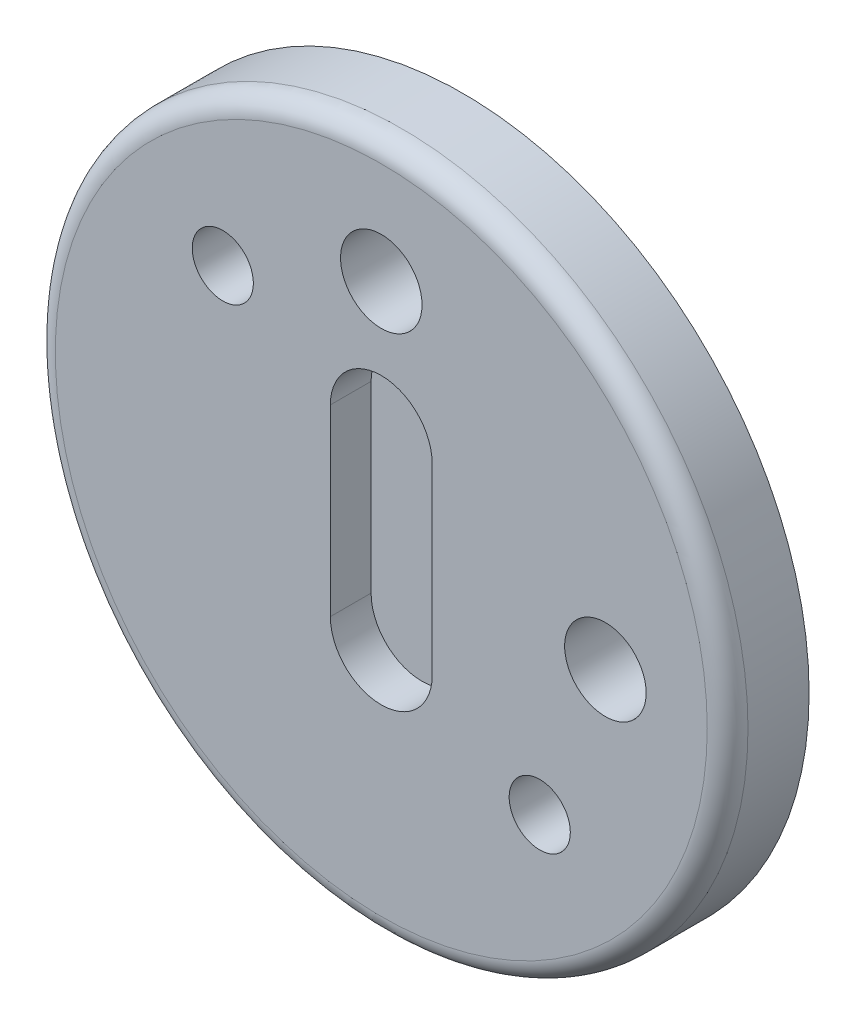
SolidWorks part; units mm, degrees
ref_plane "Front Plane" through (0, 0, 0) normal (0, 0, 1) x (1, 0, 0)
ref_plane "Top Plane" through (0, 0, 0) normal (0, 1, 0) x (1, 0, 0)
ref_plane "Right Plane" through (0, 0, 0) normal (1, 0, 0) x (0, 0, -1)
other "Configuration Table"
sketch "Sketch1" plane through (0, 0, 0) normal (0, 0, 1) x (1, 0, 0)
  circle A0 centre (0, 0) radius 17
  dimension "D1" = 34
extrude "Boss-Extrude1" add sketch "Sketch1" along normal blind 4
sketch "Sketch2" plane through (0, 0, 4) normal (0, 0, 1) x (1, 0, 0)
  line L0 (0, 4.5) -> (0, -4.5) construction
  line L1 (2.5, 4.5) -> (2.5, -4.5)
  line L2 (-2.5, 4.5) -> (-2.5, -4.5)
  arc A0 (2.5, 4.5) -> (-2.5, 4.5) centre (0, 4.5) ccw
  arc A1 (-2.5, -4.5) -> (2.5, -4.5) centre (0, -4.5) ccw
  point P3 (0, 0)
  point P9 (0, 7)
  point P10 (0, -7)
  dimension "D1" = 14
  dimension "D2" = 5
extrude "Cut-Extrude1" cut sketch "Sketch2" against normal blind 2
sketch "Sketch3" plane through (0, 0, 4) normal (0, 0, 1) x (1, 0, 0)
  line L0 (0, 0) -> (7.7782, -7.7782) construction
  line L1 (0, 0) -> (-7.7782, 7.7782) construction
  circle A0 centre (0, 0) radius 11 construction
  circle A1 centre (0, 11) radius 2
  circle A2 centre (11, 0) radius 2
  circle A3 centre (-7.7782, 7.7782) radius 1.5
  circle A4 centre (7.7782, -7.7782) radius 1.5
  dimension "D1" = 22
  dimension "D2" = 4
  dimension "D5" = 3
  dimension "D3" = 45
  dimension "D4" = 45
extrude "Cut-Extrude2" cut sketch "Sketch3" against normal blind 4
fillet "Fillet1" radius 1 1 edges at (17, 0, 4)
